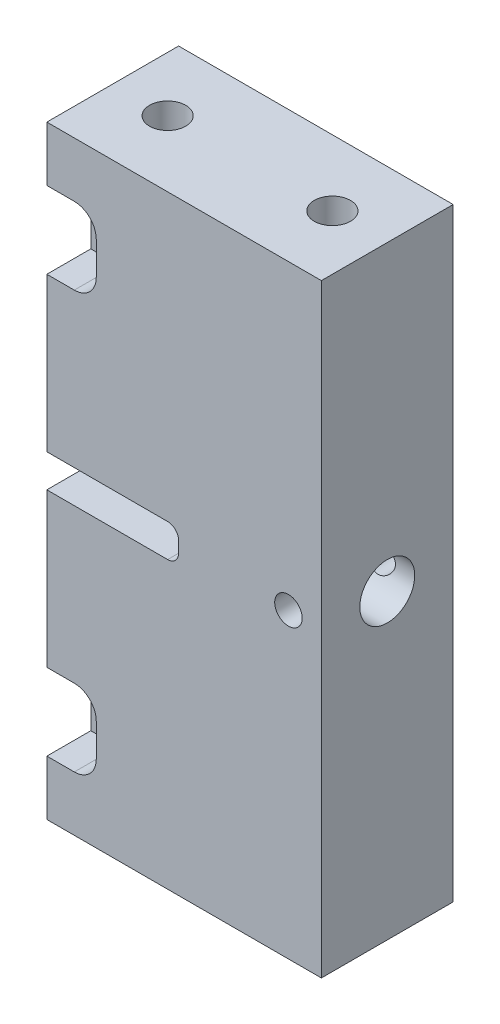
from build123d import *

# Parameters (mm, degrees)
SKETCH_1_W                  = 12
SKETCH_1_H                  = 55
EXTRUDE_1_DEPTH             = 25
SKETCH_2_R                  = 1.1
CUT_EXTRUDE_1_DEPTH         = 25
SKETCH_3_R                  = 2.5
CUT_EXTRUDE_2_DEPTH         = 8
SKETCH_4_W                  = 24
SKETCH_4_H                  = 3
CUT_EXTRUDE_3_DEPTH         = 6
HOLE_WIZARD_M4_1_AT_2_COUNT = 2
HOLE_WIZARD_M4_1_AT_2_PITCH = 15
FILLET_1_R                  = 1
CUT_EXTRUDE_4_DEPTH         = 4
HOLE_WIZARD_M3_1_D          = 2.5
FILLET_2_R                  = 1


with BuildPart() as part:
    # 草图1 → 凸台-拉伸1 (new body)
    with BuildSketch(Plane(origin=(0, 0, 0), x_dir=(0, 0, -1), z_dir=(1, 0, 0))):
        Rectangle(SKETCH_1_W, SKETCH_1_H)
    extrude(amount=EXTRUDE_1_DEPTH)

    # 草图2 → 切除-拉伸1 (cut)
    with BuildSketch(Plane(origin=(25, 0, 0), x_dir=(0, 0, -1), z_dir=(1, 0, 0))):
        Circle(SKETCH_2_R)
    extrude(amount=-CUT_EXTRUDE_1_DEPTH, mode=Mode.SUBTRACT)

    # 草图3 → 切除-拉伸2 (cut)
    with BuildSketch(Plane(origin=(25, 0, 0), x_dir=(0, 0, -1), z_dir=(1, 0, 0))):
        Circle(SKETCH_3_R)
    extrude(amount=-CUT_EXTRUDE_2_DEPTH, mode=Mode.SUBTRACT)

    # 草图4 → 切除-拉伸3 (cut)
    with BuildSketch(Plane.XY.offset(6)):
        Rectangle(SKETCH_4_W, SKETCH_4_H)
    extrude(amount=-CUT_EXTRUDE_3_DEPTH, mode=Mode.SUBTRACT)

    # 草图7 → M4 螺纹孔1 (revolve, cut)
    with BuildSketch(Plane(origin=(5, 27.5, 0), x_dir=(0, 0, 1), z_dir=(1, 0, 0))):
        Polygon((0, 0), (0, 11.091420021), (1.65, 10.1), (1.65, 0), align=None)
    hole_wizard_m4_1 = revolve(axis=Axis((5, 33.85, 0), (0, -1, 0)), mode=Mode.SUBTRACT)

    # M4 螺纹孔1 at 2: M4 螺纹孔1 ×2
    with Locations(*[(i * HOLE_WIZARD_M4_1_AT_2_PITCH, 0, 0) for i in range(1, HOLE_WIZARD_M4_1_AT_2_COUNT)]):
        add(hole_wizard_m4_1, mode=Mode.SUBTRACT)

    # 镜向1: M4 螺纹孔1 across plane
    add(hole_wizard_m4_1.mirror(Plane.ZX), mode=Mode.SUBTRACT)

    # 镜向1 copy 1 sketch → 镜向1 copy 1 (revolve, cut)
    with BuildSketch(Plane(origin=(20, -27.5, 0), x_dir=(0, 0, 1), z_dir=(1, 0, 0))):
        Polygon((0, 0), (0, -11.091420021), (1.65, -10.1), (1.65, 0), align=None)
    revolve(axis=Axis((20, -33.85, 0), (0, -1, 0)), mode=Mode.SUBTRACT)

    # 圆角1
    fillet_1_edges = [part.edges().sort_by_distance(p)[0] for p in [
        (12, -1.5, 3),
        (12, 1.5, 3),
    ]]
    fillet(fillet_1_edges, radius=FILLET_1_R)

    # 草图9 → 切除-拉伸4 (cut)
    with BuildSketch(Plane.XY.offset(6)):
        with BuildLine():
            Line((-4.5, 22.5), (2.5, 22.5))
            ThreePointArc((2.5, 22.5), (3.914213562, 21.914213562), (4.5, 20.5))
            Line((4.5, 20.5), (4.5, 17.5))
            ThreePointArc((4.5, 17.5), (3.914213562, 16.085786438), (2.5, 15.5))
            Line((2.5, 15.5), (-4.5, 15.5))
            Line((-4.5, 15.5), (-4.5, 22.5))
        make_face()
    cut_extrude_4 = extrude(amount=-CUT_EXTRUDE_4_DEPTH, mode=Mode.SUBTRACT)

    # 镜向2: 切除-拉伸4 across plane
    add(cut_extrude_4.mirror(Plane.ZX), mode=Mode.SUBTRACT)

    # M3 螺纹孔1 (through all)
    with Locations(Plane.XY.offset(6)):
        with Locations((22, 0)):
            Hole(HOLE_WIZARD_M3_1_D / 2)

    # 圆角2
    fillet_2_edges = [part.edges().sort_by_distance(p)[0] for p in [
        (17, 0, 1.1),
    ]]
    fillet(fillet_2_edges, radius=FILLET_2_R)


solid = part.part
